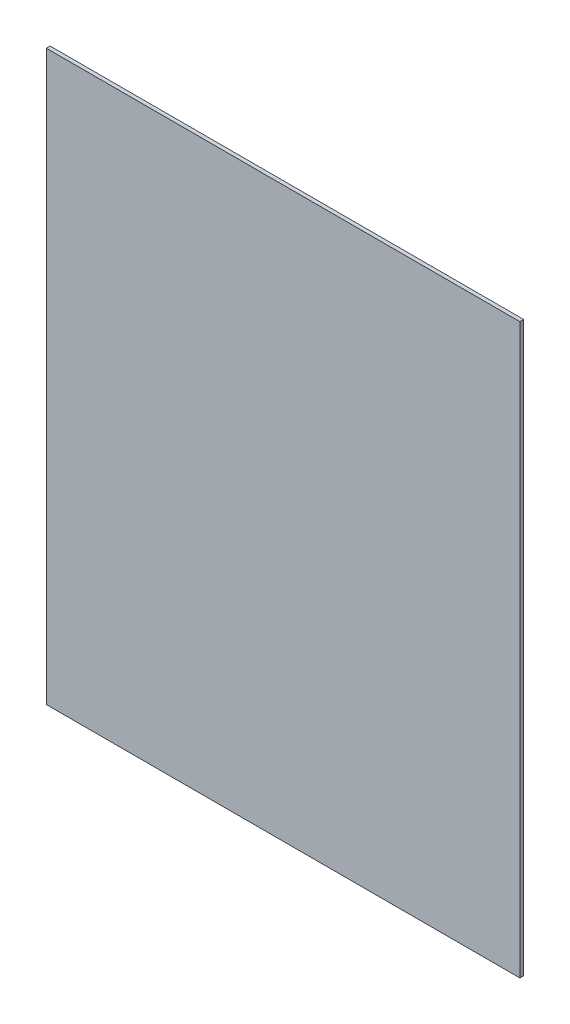
SolidWorks part; units mm, degrees
ref_plane "Front Plane" through (0, 0, 0) normal (0, 0, 1) x (1, 0, 0)
ref_plane "Top Plane" through (0, 0, 0) normal (0, 1, 0) x (1, 0, 0)
ref_plane "Right Plane" through (0, 0, 0) normal (1, 0, 0) x (0, 0, -1)
sketch "Sketch1" plane through (0, 0, 0) normal (0, 0, 1) x (1, 0, 0)
  line L1 (0, 0) -> (250, 0)
  line L2 (0, 0) -> (0, 300)
  line L3 (0, 300) -> (250, 300)
  line L4 (250, 0) -> (250, 300)
  dimension "D1" = 300
  dimension "D2" = 250
extrude "Boss-Extrude1" add sketch "Sketch1" along normal blind 2
